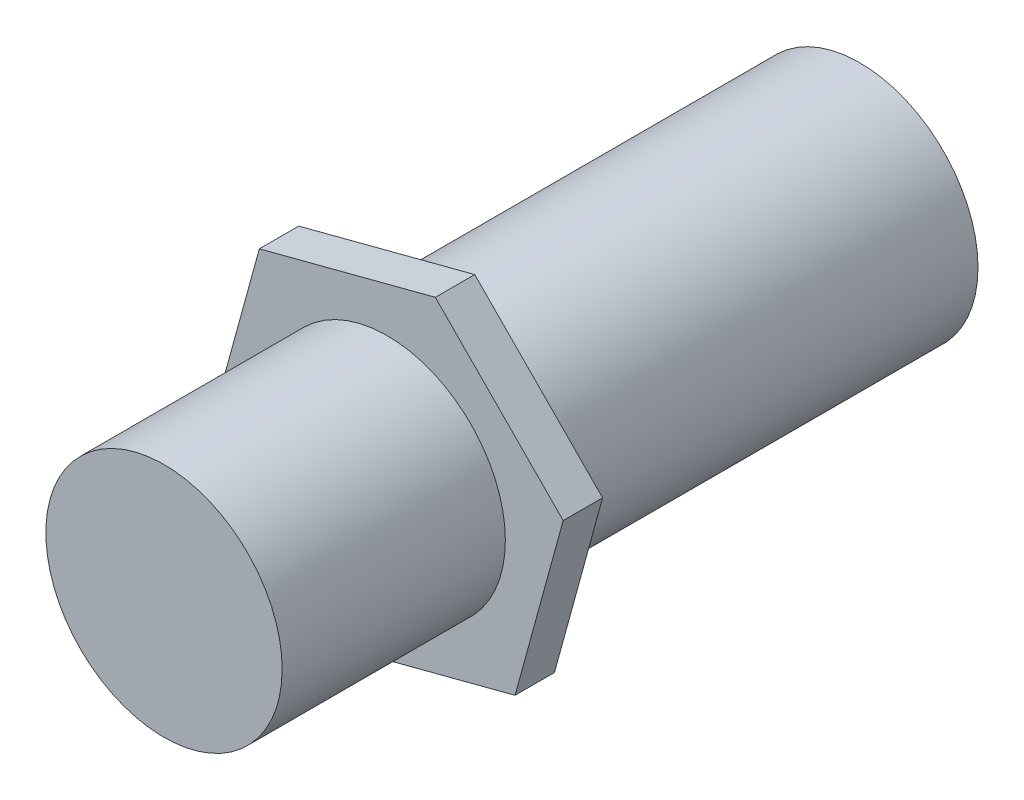
SolidWorks part; units mm, degrees
ref_plane "Front Plane" through (0, 0, 0) normal (0, 0, 1) x (1, 0, 0)
ref_plane "Top Plane" through (0, 0, 0) normal (0, 1, 0) x (1, 0, 0)
ref_plane "Right Plane" through (0, 0, 0) normal (1, 0, 0) x (0, 0, -1)
sketch "Sketch1" plane through (0, 0, 0) normal (0, 0, 1) x (1, 0, 0)
  circle A0 centre (0, 0) radius 9
extrude "Boss-Extrude1" add sketch "Sketch1" along normal blind 20 and the other way blind 33
sketch "Sketch2" plane through (0, 0, 0) normal (0, 0, 1) x (1, 0, 0)
  line L1 (9.7384, -9.8572) -> (13.4057, 3.5051)
  line L2 (13.4057, 3.5051) -> (3.6674, 13.3623)
  line L3 (3.6674, 13.3623) -> (-9.7384, 9.8572)
  line L4 (-9.7384, 9.8572) -> (-13.4057, -3.5051)
  line L5 (-13.4057, -3.5051) -> (-3.6674, -13.3623)
  line L6 (-3.6674, -13.3623) -> (9.7384, -9.8572)
  circle A1 centre (0, 0) radius 12 construction
extrude "Boss-Extrude2" add sketch "Sketch2" along normal blind 3
